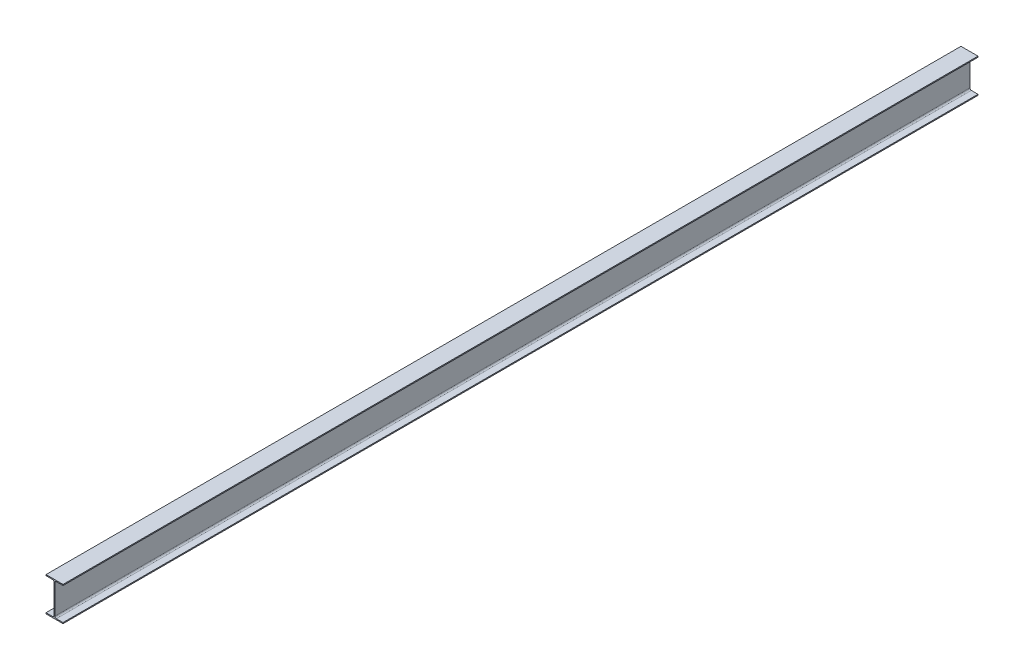
SolidWorks part; units mm, degrees
ref_plane "Front Plane" through (0, 0, 0) normal (0, 0, 1) x (1, 0, 0)
ref_plane "Top Plane" through (0, 0, 0) normal (0, 1, 0) x (1, 0, 0)
ref_plane "Right Plane" through (0, 0, 0) normal (1, 0, 0) x (0, 0, -1)
other "Configuration Table"
sketch "Sketch1" plane through (0, 0, 0) normal (0, 0, 1) x (1, 0, 0)
  line L0 (0, 0) -> (0, 300) construction
  line L1 (75, 0) -> (-75, 0)
  line L2 (-75, 0) -> (-75, 9)
  line L3 (-75, 9) -> (-16.25, 9)
  line L4 (3.25, 22) -> (3.25, 278)
  line L6 (-75, 291) -> (-75, 300)
  line L7 (-75, 300) -> (75, 300)
  line L8 (-3.25, 22) -> (-3.25, 278)
  line L9 (75, 291) -> (75, 300)
  line L10 (16.25, 291) -> (75, 291)
  line L11 (75, 9) -> (16.25, 9)
  line L12 (75, 0) -> (75, 9)
  line L13 (-16.25, 291) -> (-75, 291)
  arc A0 (16.25, 9) -> (3.25, 22) centre (16.25, 22) cw
  arc A1 (-3.25, 22) -> (-16.25, 9) centre (-16.25, 22) cw
  arc A2 (3.25, 278) -> (16.25, 291) centre (16.25, 278) cw
  arc A3 (-3.25, 278) -> (-16.25, 291) centre (-16.25, 278) ccw
  point P18 (3.25, 9)
  point P21 (-3.25, 9)
  point P24 (3.25, 291)
  point P27 (-3.25, 291)
  dimension "D6" = 13
  dimension "D1" = 300
  dimension "D2" = 150
  dimension "D3" = 6.5
  dimension "D4" = 9
  dimension "D5" = 9
extrude "Boss-Extrude1" add sketch "Sketch1" along normal blind 8060
